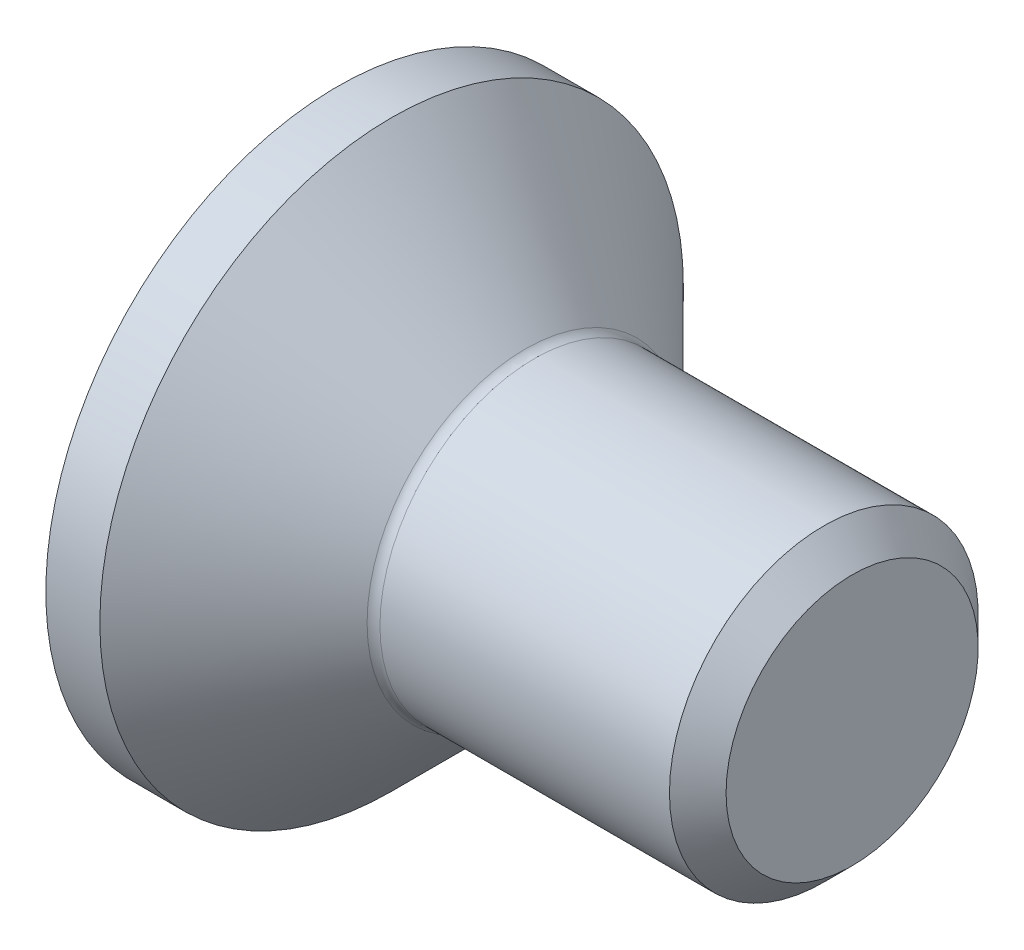
SolidWorks part; units mm, degrees
ref_plane "Front" through (0, 0, 0) normal (0, 0, 1) x (1, 0, 0)
ref_plane "Top" through (0, 0, 0) normal (0, 1, 0) x (1, 0, 0)
ref_plane "Right" through (0, 0, 0) normal (1, 0, 0) x (0, 0, -1)
other "Configuration Table"
sketch "Sketch1" plane through (0, 0, 0) normal (0, 0, 1) x (1, 0, 0)
  line L0 (0, 0) -> (0, 6.72)
  line L1 (0, 6.72) -> (3.72, 3)
  line L2 (3.72, 3) -> (10, 3)
  line L3 (10, 3) -> (10, 0)
  line L4 (10, 0) -> (0, 0)
  line L5 (-0.5871, 0) -> (5.4927, 0) construction
revolve "Base" add sketch "Sketch1" angle 360 about L5
cosmetic thread "ThreadCosmetic1" parameters "b"=4.64, "D2"=4.9
sketch "Sketch2" plane through (0, 0, 0) normal (1, 0, 0) x (0, 0, -1)
  line L1 (2.3094, 0) -> (1.1547, 2)
  line L2 (1.1547, 2) -> (-1.1547, 2)
  line L3 (-1.1547, 2) -> (-2.3094, 0)
  line L4 (-2.3094, 0) -> (-1.1547, -2)
  line L5 (-1.1547, -2) -> (1.1547, -2)
  line L6 (1.1547, -2) -> (2.3094, 0)
  circle A0 centre (0, 0) radius 2 construction
  dimension "s" = 4
extrude "HexagonSocket" cut sketch "Sketch2" along normal blind 1.1
sketch "Sketch3" plane through (0, 0, 0) normal (0, 0, 1) x (1, 0, 0)
  line L0 (-0.4391, 0) -> (4.425, 0) construction
  line L1 (1.1, 0) -> (1.1, -2) construction
  line L2 (1.1, 2) -> (2.2547, 0)
  line L3 (2.2547, 0) -> (1.1, -2) construction
  line L4 (1.1, 2) -> (1.1, 0)
  line L5 (1.1, 0) -> (2.2547, 0)
  line L7 (1.1, 2) -> (1.1, 0) construction
  dimension "D1" = 120
revolve "Cut-Revolve1" cut sketch "Sketch3" angle 360 about L0
fillet "HeadFillet" radius 0.25 1 edges at (3.72, 0, 3)
chamfer "Chamfer" distance 0.55 angle 45 1 edges at (10, 0, 3)
sketch "Sketch4" plane through (0, 0, 0) normal (0, 1, 0) x (1, 0, 0)
  line L0 (11.8531, 0) -> (-2.694, 0) construction
  line L1 (-2, 10.67) -> (3, 10.67)
  line L2 (-2, 10.67) -> (-2, 5.67)
  line L3 (-2, 5.67) -> (3, 5.67)
  line L4 (3, 10.67) -> (3, 5.67)
  line L5 (0, 6.72) -> (0, -6.72) construction
  dimension "dk" = 11.34
  dimension "D2" = 2
  dimension "D3" = 5
  dimension "D4" = 5
revolve "Cut-Revolve2" cut sketch "Sketch4" angle 360 about L0
sketch "Sketch5" plane through (0, 0, 0) normal (0, 0, 1) x (1, 0, 0)
  line L0 (9.45, 2.5237) -> (9.725, 3)
  line L1 (9.725, 3) -> (9.725, 3.55)
  line L2 (9.725, 3.55) -> (9.175, 3.55)
  line L3 (9.175, 3.55) -> (9.175, 3)
  line L4 (9.175, 3) -> (9.45, 2.5237)
  line L5 (0, 0) -> (10.6885, 0) construction
  line L6 (9.45, 3) -> (9.45, -3) construction
revolve "Cut-Revolve10" [suppressed] cut sketch "Sketch5" angle 360 about L5
pattern_linear "LPattern10" [suppressed] count 7 spacing 0.66 along (1, 0, 0)
equation "\"D1@Chamfer\" = (  \"d@Sketch1\" - \"D2@ThreadCosmetic1\" )  / 2"
equation "\"D1@Sketch5\" = \"d@Sketch1\""
equation "\"D2@Sketch5\" =  ( \"d@Sketch1\" - \"D2@ThreadCosmetic1\" )  / 2"
equation "\"D3@LPattern10\" = \"D2@Sketch5\" * 1.2"
equation "\"D1@LPattern10\" = \"b@ThreadCosmetic1\" / \"D3@LPattern10\""
